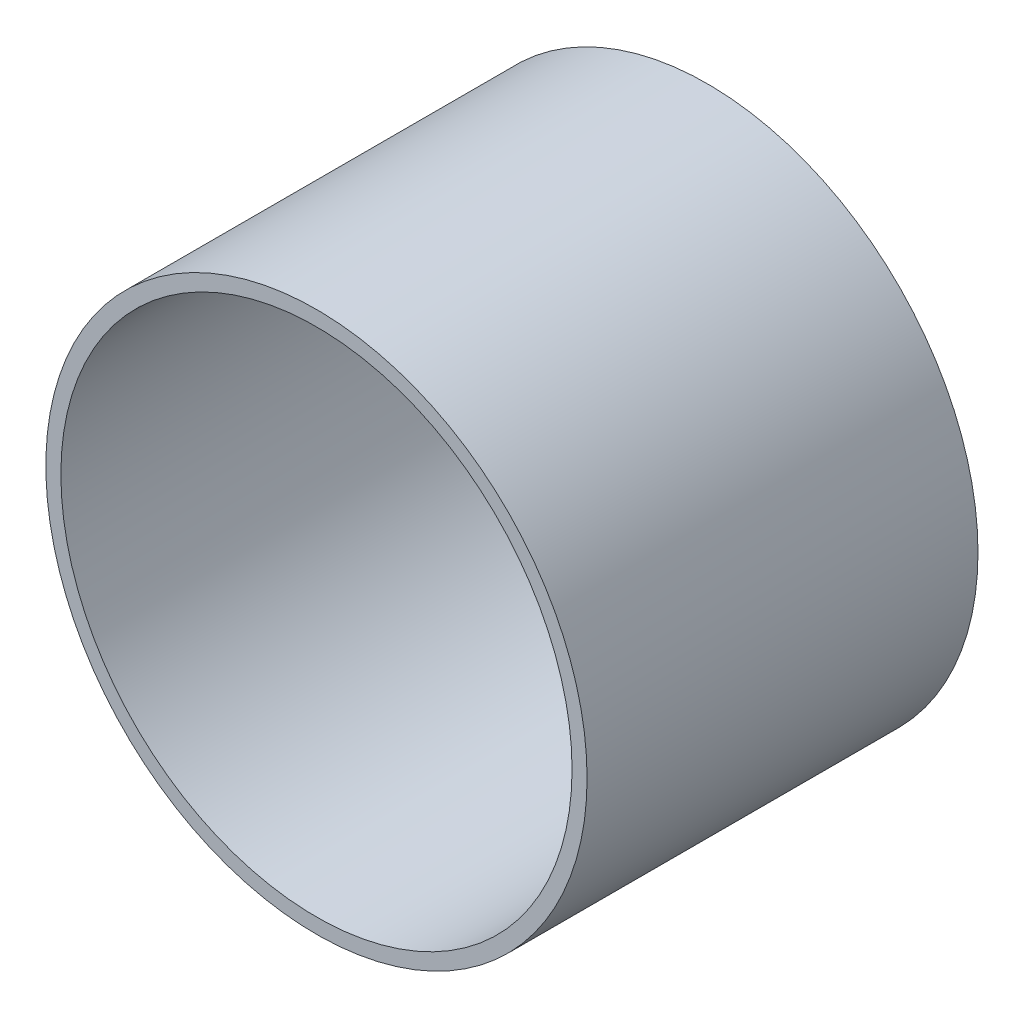
from build123d import *

# Parameters (mm, degrees)
SKETCH_1_R      = 45
SKETCH_1_R_2    = 42.5
EXTRUDE_1_DEPTH = 32.5


with BuildPart() as part:
    # 草图1 → 凸台-拉伸1 (new, symmetric)
    with BuildSketch(Plane.XY):
        Circle(SKETCH_1_R)
        Circle(SKETCH_1_R_2, mode=Mode.SUBTRACT)
    extrude(amount=EXTRUDE_1_DEPTH, both=True)


solid = part.part
